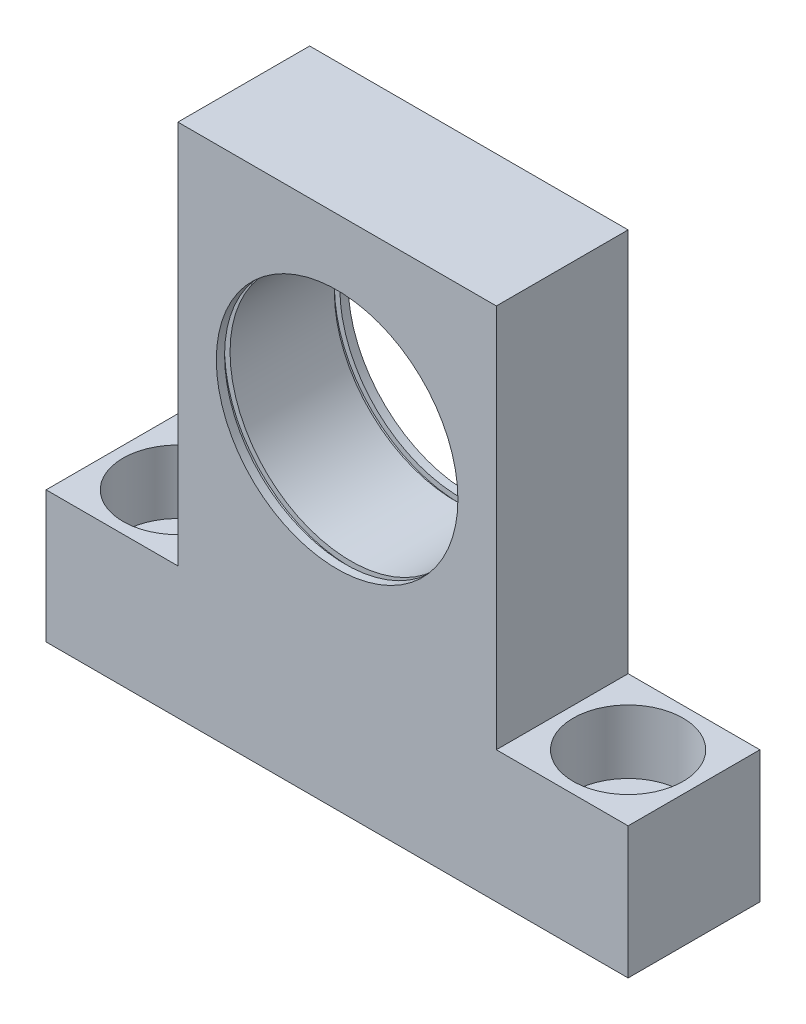
SolidWorks part; units mm, degrees
ref_plane "前视基准面" through (0, 0, 0) normal (0, 0, 1) x (1, 0, 0)
ref_plane "上视基准面" through (0, 0, 0) normal (0, 1, 0) x (1, 0, 0)
ref_plane "右视基准面" through (0, 0, 0) normal (1, 0, 0) x (0, 0, -1)
sketch "草图1" plane through (0, 0, 0) normal (0, 0, 1) x (1, 0, 0)
  line L0 (-16.2697, -16.0377) -> (36.7303, -16.0377)
  line L5 (36.7303, -16.0377) -> (36.7303, -4.0377)
  line L6 (36.7303, -4.0377) -> (24.7303, -4.0377)
  line L7 (24.7303, -4.0377) -> (24.7303, 30.9623)
  line L8 (24.7303, 30.9623) -> (-4.2697, 30.9623)
  line L9 (-4.2697, 30.9623) -> (-4.2697, -4.0377)
  line L10 (-4.2697, -4.0377) -> (-16.2697, -4.0377)
  line L11 (-16.2697, -4.0377) -> (-16.2697, -16.0377)
  circle A0 centre (10.2303, 13.9623) radius 11
  dimension "D7" = 22
  dimension "D1" = 53
  dimension "D2" = 12
  dimension "D3" = 12
  dimension "D4" = 12
  dimension "D5" = 12
  dimension "D6" = 35
  dimension "D8" = 17
  dimension "D9" = 14.5
extrude "凸台-拉伸1" add sketch "草图1" along normal blind 12
sketch "草图2" plane through (0, -4.0377, 0) normal (0, 1, 0) x (1, 0, 0)
  line L0 (-4.2697, 0) -> (-16.2697, 0) construction
  line L1 (-16.2697, -12) -> (-16.2697, 0) construction
  line L2 (36.7303, -12) -> (36.7303, 0) construction
  line L3 (36.7303, 0) -> (24.7303, 0) construction
  circle A0 centre (-10.2697, -6) radius 2.75
  circle A1 centre (30.7303, -6) radius 2.75
  dimension "D1" = 5.5
  dimension "D2" = 5.5
  dimension "D3" = 6
  dimension "D4" = 6
  dimension "D5" = 6
  dimension "D6" = 6
extrude "切除-拉伸1" cut sketch "草图2" against normal through all
sketch "草图3" plane through (0, -4.0377, 0) normal (0, 1, 0) x (1, 0, 0)
  circle A0 centre (-10.2697, -6) radius 5
  circle A1 centre (30.7303, -6) radius 5
  dimension "D1" = 10
  dimension "D2" = 10
extrude "切除-拉伸2" cut sketch "草图3" against normal blind 5.8
ref_plane "基准面1" through (0, 0, 11) normal (0, 0, 1) x (1, 0, 0)
sketch "草图4" plane through (0, 0, 11) normal (0, 0, 1) x (1, 0, 0)
  circle A0 centre (10.2303, 13.9623) radius 11.5
  dimension "D1" = 23
extrude "切除-拉伸3" cut sketch "草图4" against normal mid plane 0.5
ref_plane "基准面2" through (0, 0, 1) normal (0, 0, -1) x (-1, 0, 0)
sketch "草图5" plane through (0, 0, 1) normal (0, 0, -1) x (-1, 0, 0)
  circle A0 centre (-10.2303, 13.9623) radius 11.5
  dimension "D1" = 23
extrude "切除-拉伸4" cut sketch "草图5" against normal mid plane 0.5
